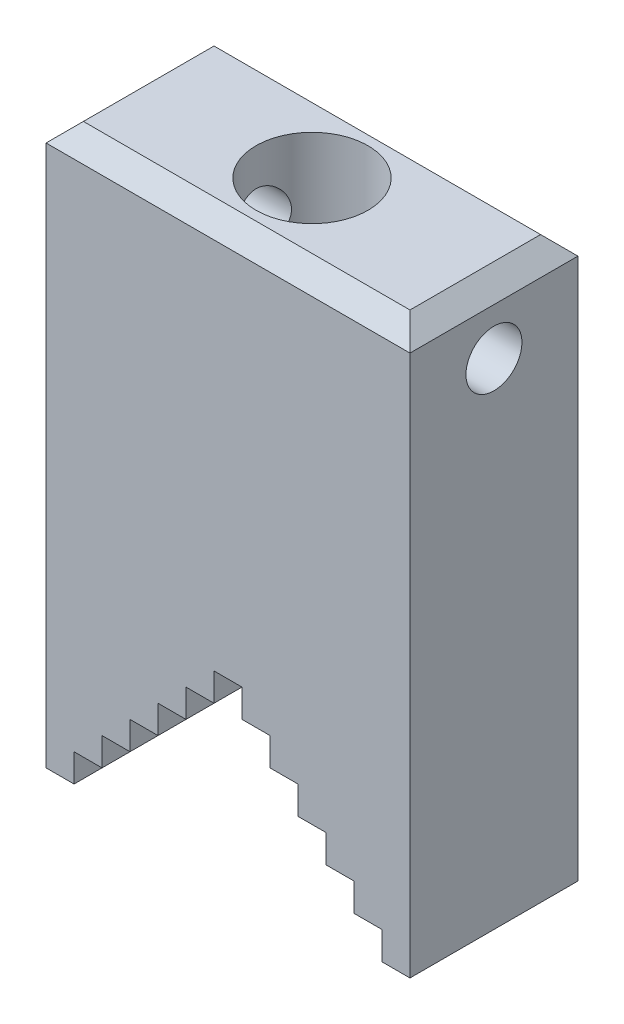
SolidWorks part; units mm, degrees
ref_plane "Front Plane" through (0, 0, 0) normal (0, 0, 1) x (1, 0, 0)
ref_plane "Top Plane" through (0, 0, 0) normal (0, 1, 0) x (1, 0, 0)
ref_plane "Right Plane" through (0, 0, 0) normal (1, 0, 0) x (0, 0, -1)
sketch "Sketch1" plane through (0, 0, 0) normal (0, 0, 1) x (1, 0, 0)
  line L0 (-16.5, -30) -> (-16.5, -27)
  line L1 (-19.5, 30) -> (19.5, 30)
  line L2 (-19.5, 30) -> (-19.5, -30)
  line L3 (-19.5, -30) -> (-16.5, -30)
  line L4 (19.5, 30) -> (19.5, -30)
  line L5 (-19.5, 30) -> (19.5, -30) construction
  line L6 (-19.5, -30) -> (19.5, 30) construction
  line L7 (-16.5, -27) -> (-13.5, -27)
  line L8 (-13.5, -27) -> (-13.5, -24)
  line L9 (-13.5, -24) -> (-10.5, -24)
  line L10 (-10.5, -24) -> (-10.5, -21)
  line L11 (-10.5, -21) -> (-7.5, -21)
  line L12 (-7.5, -21) -> (-7.5, -18)
  line L13 (-7.5, -18) -> (-4.5, -18)
  line L14 (-4.5, -18) -> (-4.5, -15)
  line L15 (-4.5, -15) -> (-1.5, -15)
  line L16 (-1.5, -15) -> (-1.5, -12)
  line L17 (0, 0) -> (0, -7.5481) construction
  line L18 (1.5, -15) -> (1.5, -12)
  line L19 (4.5, -15) -> (1.5, -15)
  line L20 (4.5, -18) -> (4.5, -15)
  line L21 (7.5, -18) -> (4.5, -18)
  line L22 (7.5, -21) -> (7.5, -18)
  line L23 (10.5, -21) -> (7.5, -21)
  line L24 (10.5, -24) -> (10.5, -21)
  line L25 (13.5, -24) -> (10.5, -24)
  line L26 (13.5, -27) -> (13.5, -24)
  line L27 (16.5, -27) -> (13.5, -27)
  line L28 (16.5, -30) -> (16.5, -27)
  line L29 (-1.5, -12) -> (1.5, -12)
  line L30 (16.5, -30) -> (19.5, -30)
  point P0 (0, 0)
  dimension "D1" = 60
  dimension "D2" = 39
  dimension "D3" = 3
  dimension "D4" = 3
extrude "Boss-Extrude1" add sketch "Sketch1" along normal mid plane 18
chamfer "Chamfer1" distance 2 angle 45 4 edges at (19.5, 30, 0) (0, 30, -9) (-19.5, 30, 0) (0, 30, 9)
sketch "Sketch2" plane through (19.5, 0, 0) normal (1, 0, 0) x (0, 0, -1)
  line L0 (-7, 30) -> (7, 30) construction
  circle A0 centre (0, 23) radius 3
  dimension "D1" = 6
  dimension "D2" = 7
extrude "Cut-Extrude1" cut sketch "Sketch2" against normal through all
sketch "Sketch3" plane through (0, 0, 0) normal (0, 0, 1) x (1, 0, 0)
  line L0 (0, 31.7281) -> (0, 9.9861) construction
  line L1 (0, 30) -> (6, 30)
  line L2 (-17.5, 30) -> (17.5, 30) construction
  line L3 (6, 30) -> (6, 10)
  line L4 (6, 10) -> (0, 6.5359)
  line L5 (0, 6.5359) -> (0, 30)
  dimension "D1" = 20
  dimension "D2" = 6
  dimension "D3" = 60
revolve "Cut-Revolve1" cut sketch "Sketch3" angle 360 about L0
